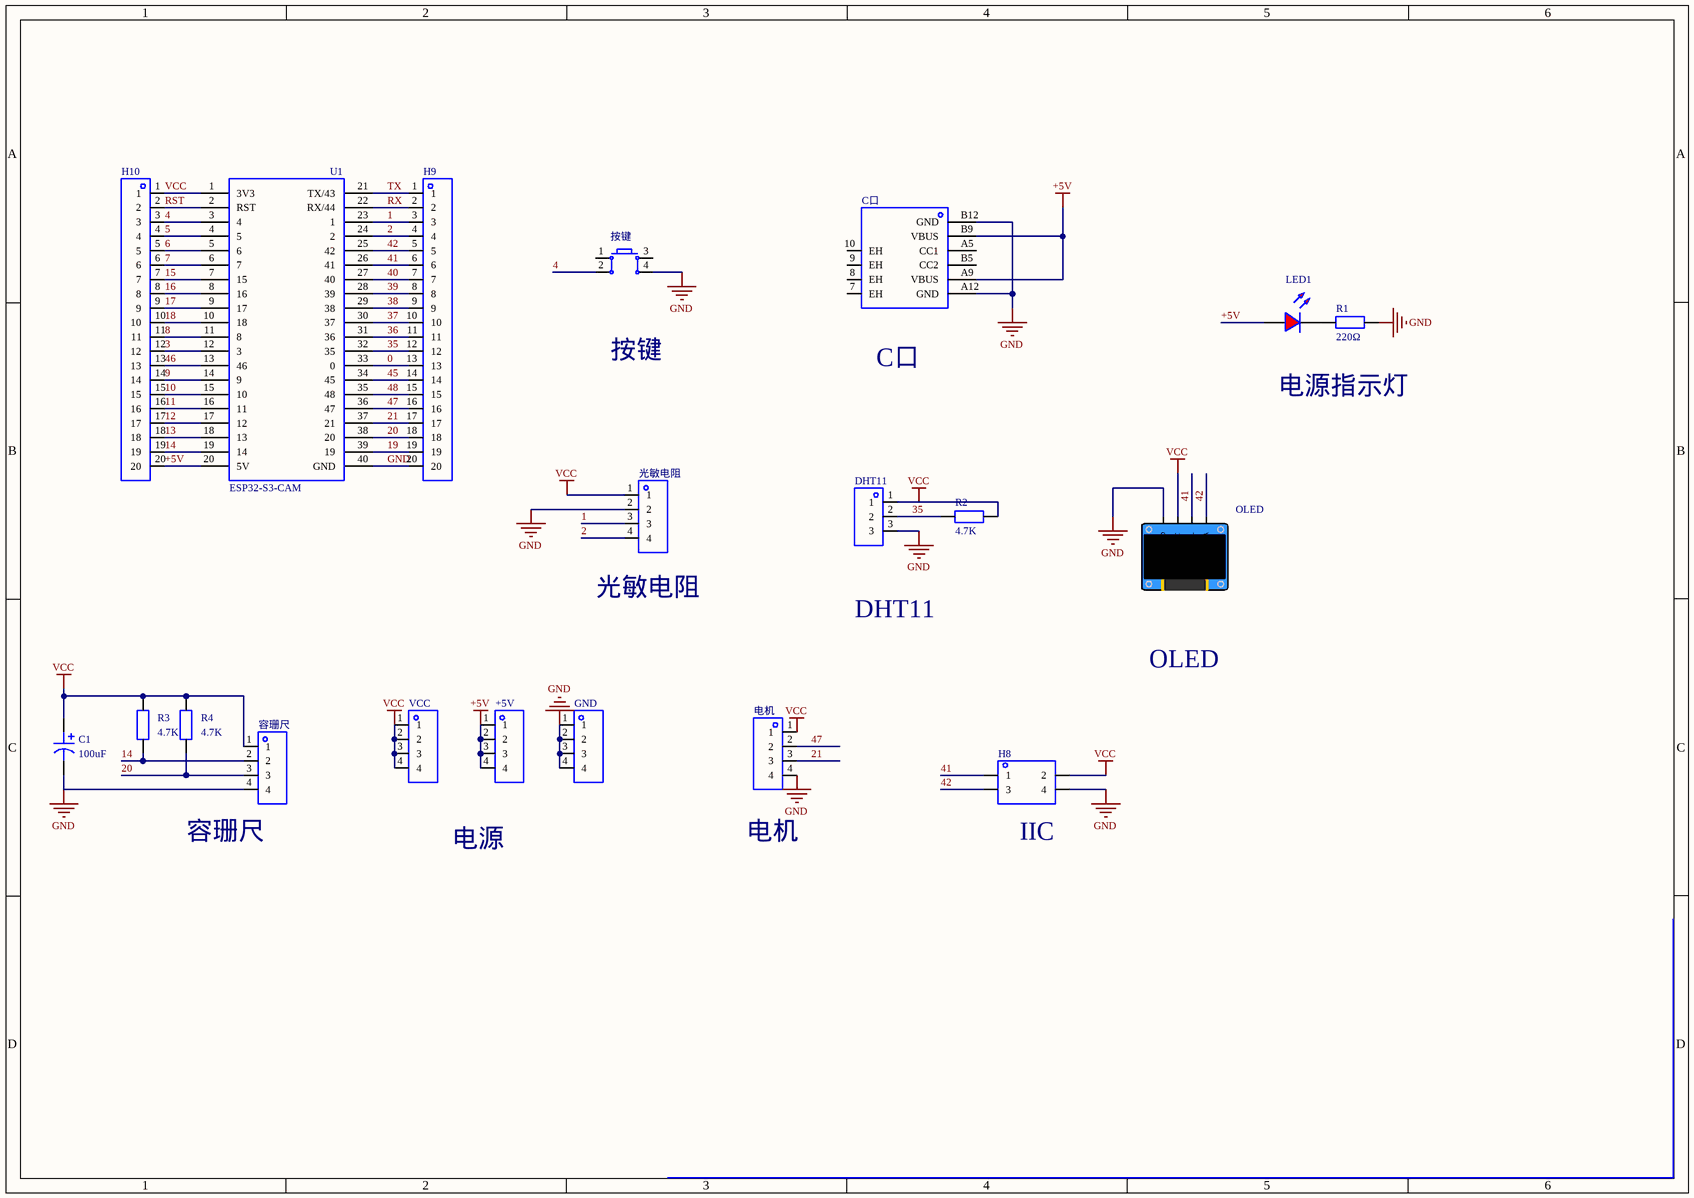
[diagram p0: MISC51152-3.schdoc]
# Altium project MISC51152-2.PrjPcb
1 sheet, 20 parts. Net scope: global (net labels, ports and power ports of the same name join across sheets).
Board file: MISC51152.pcbdoc

## Sheet MISC51152-3.schdoc
size 297 x 209 mm; Version: V1.0; @Project Name: MISC51152; @Page Count: 1; @Update Date: 2026-05-18; @Create Date: 2026-05-18; @Schematic Name: MISC51152; @Page No: 1; @Create Time: 23:22:16; @Update Time: 17:32:40; @Board Name: MISC51152

### Parts
+5V  (no value)  [HDR-TH_4P-P2.54-V-F]
C1  100uF  [CAP-TH_BD8.0-P3.50-D0.6-FD_1]
C口  (no value)  [USB_ TYPE-C-6P]
DHT11  (no value)  [HDR-TH_3P-P2.54-V-F]
GND  (no value)  [HDR-TH_4P-P2.54-V-F]
H8  (no value)  [HDR-TH_4P-P2.54-V-F-R2-C2-S2.54]
H9  (no value)  [HDR-TH_20P-P2.54-V-M-1]
H10  (no value)  [HDR-TH_20P-P2.54-V-M-1]
LED1  (no value)  [LED_TH-3mm]
OLED  (no value)  [0.96OLED_4P]
R1  220Ω  [Res_1/8W]
R2  4.7K  [Res_1/8W]
R3  4.7K  [Res_1/8W]
R4  4.7K  [Res_1/8W]
U1  (no value)  [ESP32-S3-CAM]
VCC  (no value)  [HDR-TH_4P-P2.54-V-F]
光敏电阻  (no value)  [HDR-TH_4P-P2.54-V-F]
容珊尺  (no value)  [HDR-TH_4P-P2.54-V-F]
按键  (no value)  [SW-TH_4P-L6.0-W6.0-P4.50-LS6.5]
电机  (no value)  [HDR-TH_4P-P2.54-V-F]

### Nets
+5V: +5V.1 +5V.2 +5V.3 +5V.4 C口.A9(VBUS) C口.B9(VBUS) H10.20 LED1.1(C) U1.20(5V)
GND: C1.2 C口.A12(GND) C口.B12(GND) DHT11.3 GND.1 GND.2 GND.3 GND.4 H8.4 H9.20 OLED.1(GND) R1.2 U1.40(GND) 光敏电阻.2 容珊尺.4 按键.4 电机.4
VCC: C1.1 DHT11.1 H8.2 H10.1 OLED.2(VCC) R2.2 R3.2 R4.2 U1.1(3V3) VCC.1 VCC.2 VCC.3 VCC.4 光敏电阻.1 容珊尺.1 电机.1
0: H9.13 U1.33(0)
1: H9.3 U1.23(1) 光敏电阻.3
2: H9.4 U1.24(2) 光敏电阻.4
3: H10.12 U1.12(3)
4: H10.3 U1.3(4) 按键.2
5: H10.4 U1.4(5)
6: H10.5 U1.5(6)
7: H10.6 U1.6(7)
8: H10.11 U1.11(8)
9: H10.14 U1.14(9)
10: H10.15 U1.15(10)
11: H10.16 U1.16(11)
12: H10.17 U1.17(12)
13: H10.18 U1.18(13)
14: H10.19 R3.1 U1.19(14) 容珊尺.2
15: H10.7 U1.7(15)
16: H10.8 U1.8(16)
17: H10.9 U1.9(17)
18: H10.10 U1.10(18)
19: H9.19 U1.39(19)
20: H9.18 R4.1 U1.38(20) 容珊尺.3
21: H9.17 U1.37(21) 电机.3
35: DHT11.2 H9.12 R2.1 U1.32(35)
36: H9.11 U1.31(36)
37: H9.10 U1.30(37)
38: H9.9 U1.29(38)
39: H9.8 U1.28(39)
40: H9.7 U1.27(40)
41: H8.1 H9.6 OLED.3(SCL) U1.26(41)
42: H8.3 H9.5 OLED.4(SDA) U1.25(42)
45: H9.14 U1.34(45)
46: H10.13 U1.13(46)
47: H9.16 U1.36(47) 电机.2
48: H9.15 U1.35(48)
RST: H10.2 U1.2(RST)
RX: H9.2 U1.22(RX/44)
TX: H9.1 U1.21(TX/43)
NetLED1_2: LED1.2(A) R1.1

Not connected (* = marked no-connect by the designer): C口 7(EH) 8(EH) 9(EH) 10(EH) A5(CC1) B5(CC2); 按键 1 3

### Notes on the sheet
- 按键
- (near C口) C口
- 电源指示灯
- (near 光敏电阻) 光敏电阻
- DHT11
- OLED
- (near 容珊尺) 容珊尺
- 电源
- (near 电机) 电机
- (near H8) IIC

### Library data of the parts
+5V GND VCC 光敏电阻 电机 = HDR-F_2.54_1x4P: Symbol: 2.54-1*4P母; ConvertToPcb: yes; ModelId: d187812051054f85879fcaa51a310d8e0819f05c4eef4c71ace90d822a990e87; ModelTransform: 419.6842,98.464,0,0,0,0,0,0,-118.11; Device: HDR-F_2.54_1x4P; AddInBom: yes; SupplierPart: C2718488; Supplier Footprint: 插件; FootprintName: HDR-TH_4P-P2.54-V-F; ModelName: HDR-TH_4P-P2.54-V-F
C1 = 100uF: Symbol: 100UF_C9900016884; AddInBom: yes; ModelId: 5fc21599cab34df2ad7753b19b2f52860819f05c4eef4c71ace90d822a990e87; ModelTransform: 315.365,314.914,0,0,0,0,0,0,-196.85; Device: 100uF; LCSC Part Name: 100uF; SupplierPart: C9900016884; ManufacturerPart: 100uF; Supplier Footprint: CAP-TH_BD8.0-P3.50-D1.0-FD; JLCPCB Part Class: Extended Part; Supplier: LCSC; ConvertToPcb: yes; FootprintName: CAP-TH_BD8.0-P3.50-D0.6-FD_1; ModelName: CAP-TH_BD8.0-P3.50-D0.6-FD_1
C口 = USB_ Type-C-6P: AddInBom: yes; ModelId: d4f492a4e6024845a13b3f6a4ef2d2cb0819f05c4eef4c71ace90d822a990e87; ModelName: USB-SMD_U262-061N-4BVC11; ModelTransform: 352.362,281.496,0,0,0,0,0,-47.244,-39.37; Symbol: USB_ TYPE-C-6P; Device: USB_ Type-C-6P; Supplier Footprint: SMD; ConvertToPcb: yes; FootprintName: USB_ TYPE-C-6P
DHT11 = HDR-F_2.54_1x3P: Symbol: PM254V-11-03-H85; ConvertToPcb: yes; ModelId: f3b3cc5aae9641bf9e56fc160cef875b; ModelName: HDR2.54-F-LI-1X3P; ModelTransform: 299.9994,100,0,0,0,0,0,0,-118.11; Device: HDR-F_2.54_1x3P; FootprintName: HDR-TH_3P-P2.54-V-F; AddInBom: yes; SupplierPart: C541850; Supplier Footprint: 插件
H8 = HDR-F_2.54_2x2: Symbol: HDR-F-2.54_2x2; ConvertToPcb: yes; ModelId: 870c884146ee4765973edc845f10b7af0819f05c4eef4c71ace90d822a990e87; ModelName: HDR-TH_4P-P2.54-F-LI-2X2P; ModelTransform: 215.7476,196.85,0,0,0,0,0,0,-118.11; Device: HDR-F_2.54_2x2; AddInBom: yes; SupplierPart: C92273; Supplier Footprint: 插件; FootprintName: HDR-TH_4P-P2.54-V-F-R2-C2-S2.54
H9 H10 = HDR-M_2.54_1x20P: 间距:2.54mm;总PIN位数:20;排数:1;插针结构:-;行距:-;安装类型:直插;圆针/方针:-;额定电流:-;额定电压:-;配合针长度:-;塑高:-;触头材质:黄铜;触头镀层:-;颜色:黑色;; Symbol: HDR_2.54-1x20P; ConvertToPcb: yes; ModelId: f68709be121d406db68b06f32a5953890819f05c4eef4c71ace90d822a990e87; ModelName: HDR-M-2.54_1x20; ModelTransform: 1999.996,100,0,0,0,0,0,0,-118.11; Device: HDR-M_2.54_1x20P; AddInBom: yes; SupplierPart: C50981; Supplier Footprint: 插件; FootprintName: HDR-TH_20P-P2.54-V-M-1
LED1 = LED_TH-R_3mm: ConvertToPcb: yes; ModelId: a497c992633541038a38947cdc58012f0819f05c4eef4c71ace90d822a990e87; ModelName: LED-TH-3mm_R; ModelTransform: 141.274,153.327,0,0,0,0,-5.984,0,-137.795; Symbol: LED_TH-R; Device: LED_TH-R_3mm; AddInBom: yes; FootprintName: LED_TH-3mm; Supplier Footprint: 插件
OLED = 0.96OLED模块_4P: ConvertToPcb: yes; ModelId: 79c000fdb68d45a296c2e9bedf4f9055; ModelTransform: 1393.69792,1318.895,0,0,0,0,0,-560.079,-137.795; Symbol: 0.96OLED模块_4P; Device: 0.96OLED模块_4P; AddInBom: yes; FootprintName: 0.96OLED_4P; Supplier Footprint: 插件; ModelName: 0.96OLED_4P
R1 = Res_AXIAL-1/8W: Symbol: 电阻; ConvertToPcb: yes; ModelId: b2b5ae7ae4c642178fe0039925c86a3f0819f05c4eef4c71ace90d822a990e87; ModelName: RES-TH_BD1.8-L3.2-P7.20-D0.4; ModelTransform: 282.86,66.88,253.09,0,0,0,0,0,-191; Device: Res_AXIAL-1/8W; Value: 220Ω; AddInBom: yes; Supplier Footprint: 轴向引线; FootprintName: Res_1/8W
R2-R4 = Res_0603: Symbol: 电阻; 3D Model: fc143cca1e79419f9cd78b61e9279f080819f05c4eef4c71ace90d822a990e87; 3D Model Transform: 31.8897,63.7794,0,90,0,0,0,0,0; ConvertToPcb: yes; ModelName: R0603; Device: Res_0603; Supplier Footprint: 0603; Value: 4.7K; AddInBom: yes; FootprintName: Res_1/8W
U1 = ESP32-S3-CAM: AddInBom: yes; Symbol: ESP32-S3-CAM; Device: ESP32-S3-CAM; ConvertToPcb: yes; FootprintName: ESP32-S3-CAM
容珊尺 = HDR-F_2.54_1x4P: Symbol: 2.54-1*4P母; 3D Model: d187812051054f85879fcaa51a310d8e0819f05c4eef4c71ace90d822a990e87; 3D Model Transform: 419.6842,98.464,0,0,0,0,0,0,-118.11; ConvertToPcb: yes; Device: HDR-F_2.54_1x4P; Supplier Part: C2718488; Supplier Footprint: 插件; FootprintName: HDR-TH_4P-P2.54-V-F; AddInBom: yes; ModelName: HDR-TH_4P-P2.54-V-F
按键 = Key_TH_6x6x6: 触点电流:50mA;额定电压(DC):12V;绝缘电阻:100MΩ;电路结构:单刀单掷;安装方式:直插;按钮形状:圆形按钮;按钮/盖帽颜色:黑色;作用力:260gf@±30gf;工作温度:-25℃~+70℃;引脚样式:PC引脚;开关长度:6mm;开关宽度:6mm;开关高度:6mm;带支架:否;; Symbol: 轻触按键; AddInBom: yes; ModelId: 20eee248bc684ccd8cbdbb1d0d91ec6f0819f05c4eef4c71ace90d822a990e87; ModelName: SW-TH_4P-L6.0-W6.0-H5.0-LS6.5-P4.50; ModelTransform: 236.22,323.03,0,90,0,0,0,0,-137.795; Device: Key_TH_6x6x6; ConvertToPcb: yes; FootprintName: SW-TH_4P-L6.0-W6.0-P4.50-LS6.5; Supplier Footprint: 插件